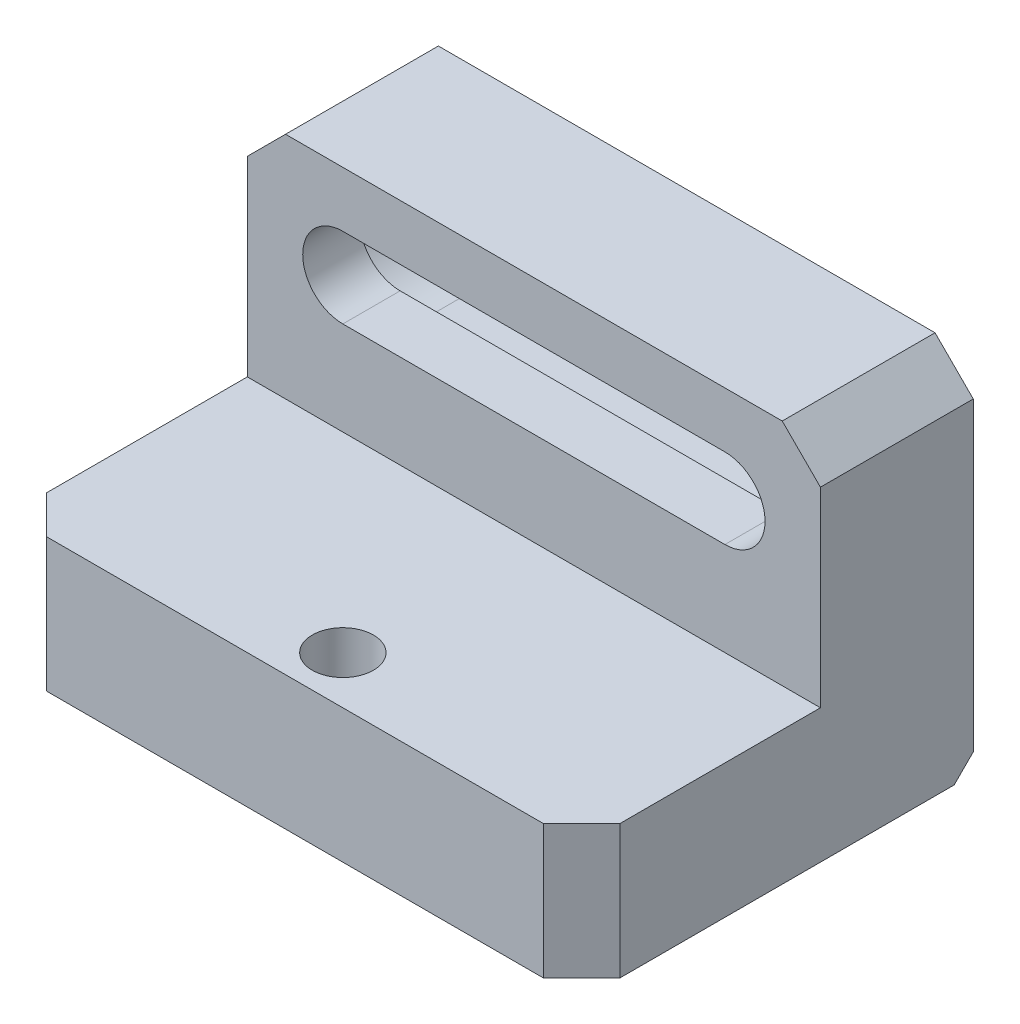
from build123d import *

# Parameters (mm, degrees)
SKETCH_1_W                = 30
SKETCH_1_H                = 19
EXTRUDE_1_DEPTH           = 20.5
SKETCH_2_W                = 30
SKETCH_2_H                = 12
CUT_EXTRUDE_1_DEPTH       = 12.5
CUT_EXTRUDE_2_DEPTH       = 28.120103245
CUT_EXTRUDE_3_DEPTH       = 5
SKETCH_5_R                = 1.75
CUT_EXTRUDE_4_DEPTH       = 10
HOLE_WIZARD_M3_1_D        = 3.2
HOLE_WIZARD_M3_1_2_REACH  = 22.628
HOLE_WIZARD_M3_1_2_BORE_R = 1.25
CHAMFER_1_SIZE            = 2
CHAMFER_2_SIZE            = 1


with BuildPart() as part:
    # 草图1 → 凸台-拉伸1 (new body)
    with BuildSketch(Plane.XY):
        Rectangle(SKETCH_1_W, SKETCH_1_H)
    extrude(amount=EXTRUDE_1_DEPTH)

    # 草图2 → 切除-拉伸1 (cut)
    with BuildSketch(Plane.XY.offset(20.5)):
        with Locations((0, 3.5)):
            Rectangle(SKETCH_2_W, SKETCH_2_H)
    extrude(amount=-CUT_EXTRUDE_1_DEPTH, mode=Mode.SUBTRACT)

    # 草图3 → 切除-拉伸2 (cut, through all)
    with BuildSketch(Plane(origin=(0, 0, 0), x_dir=(-1, 0, 0), z_dir=(0, 0, -1))):
        with BuildLine():
            Line((10, 2.4), (-10, 2.4))
            ThreePointArc((-10, 2.4), (-12.1, 4.5), (-10, 6.6))
            Line((-10, 6.6), (10, 6.6))
            ThreePointArc((10, 6.6), (12.1, 4.5), (10, 2.4))
        make_face()
    extrude(amount=-CUT_EXTRUDE_2_DEPTH, mode=Mode.SUBTRACT)

    # 草图4 → 切除-拉伸3 (cut)
    with BuildSketch(Plane(origin=(0, 0, 0), x_dir=(-1, 0, 0), z_dir=(0, 0, -1))):
        with BuildLine():
            Line((10, 0.5), (-10, 0.5))
            ThreePointArc((-10, 0.5), (-14, 4.5), (-10, 8.5))
            Line((-10, 8.5), (10, 8.5))
            ThreePointArc((10, 8.5), (14, 4.5), (10, 0.5))
        make_face()
    extrude(amount=-CUT_EXTRUDE_3_DEPTH, mode=Mode.SUBTRACT)

    # 草图5 → 切除-拉伸4 (cut)
    with BuildSketch(Plane(origin=(0, 0, 0), x_dir=(-1, 0, 0), z_dir=(0, 0, -1))):
        with Locations((0, -6)):
            Circle(SKETCH_5_R)
    extrude(amount=-CUT_EXTRUDE_4_DEPTH, mode=Mode.SUBTRACT)

    # Hole Wizard M3 _1 (through all)
    with Locations(Plane(origin=(0, -9.5, 0), x_dir=(-1, 0, 0), z_dir=(0, -1, 0))):
        with Locations((0, -18)):
            Hole(HOLE_WIZARD_M3_1_D / 2)

    # Hole Wizard M3 _1 2 bore → Hole Wizard M3 _1 2 (cut, up to next)
    with BuildSketch(Plane(origin=(0, 0, 10), x_dir=(-1, 0, 0), z_dir=(0, 0, -1)), mode=Mode.PRIVATE) as hole_wizard_m3_1_2_sk1:
        with Locations((0, -6)):
            Circle(HOLE_WIZARD_M3_1_2_BORE_R)
    hole_wizard_m3_1_2_tool1 = extrude(hole_wizard_m3_1_2_sk1.sketch, amount=-HOLE_WIZARD_M3_1_2_REACH, mode=Mode.PRIVATE) & part.part
    add(hole_wizard_m3_1_2_tool1.solids().sort_by_distance((0, -6, 10))[0], mode=Mode.SUBTRACT)

    # 倒角1
    chamfer_1_edges = [part.edges().sort_by_distance(p)[0] for p in [
        (-15, -6, 20.5),
        (-15, 9.5, 4),
        (15, 9.5, 4),
        (15, -6, 20.5),
    ]]
    chamfer(chamfer_1_edges, length=CHAMFER_1_SIZE)

    # 倒角2
    chamfer_2_edges = [part.edges().sort_by_distance(p)[0] for p in [
        (0, -9.5, 0),
    ]]
    chamfer(chamfer_2_edges, length=CHAMFER_2_SIZE)


solid = part.part
